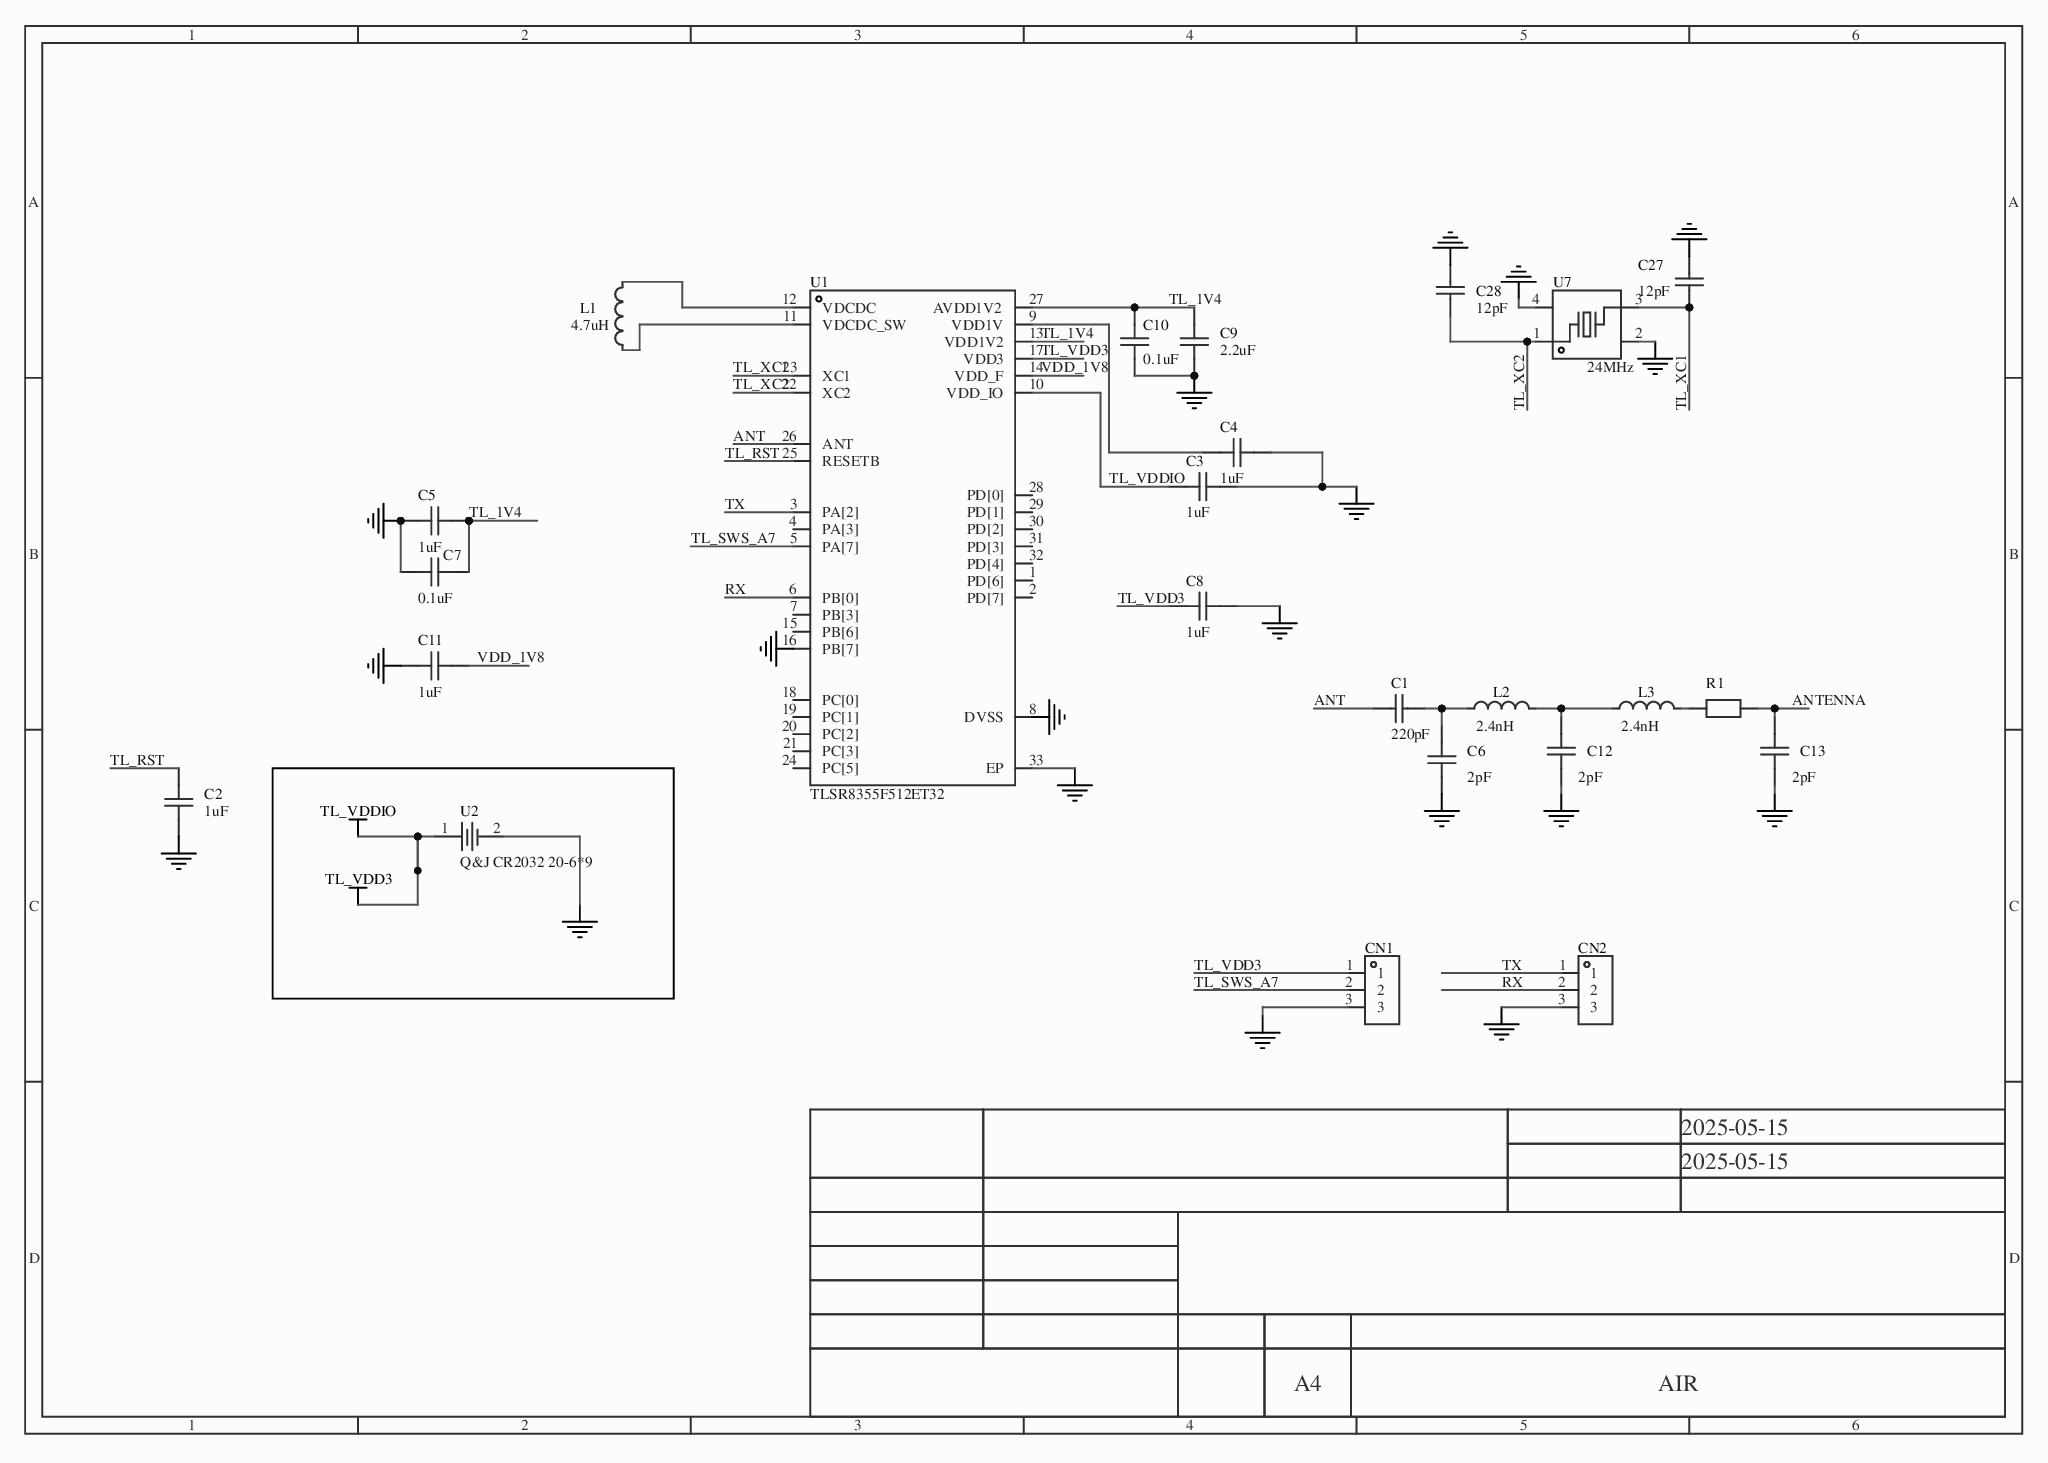
[diagram p0: MISC79017-2.schdoc]
# Altium project MISC79017-6.PrjPCB
1 sheet, 24 parts. Net scope: global (net labels, ports and power ports of the same name join across sheets).
Board file: MISC79017.PcbDoc

## Sheet MISC79017-2.schdoc
size 307 x 218 mm; Version: V1.0; @Page Count: 1; @Update Date: 2025-05-15; @Create Date: 2025-05-15; @Schematic Name: MISC79017; @Page No: 1; @Create Time: 16:34:02; @Update Time: 16:34:04

### Parts
C1  220pF  [C0402]
C2  1uF  [C0402]
C3  1uF  [C0402]
C4  1uF  [C0402]
C5  1uF  [C0402]
C6  2pF  [C0402]
C7  0.1uF  [C0603]
C8  1uF  [C0402]
C9  2.2uF  [C0402]
C10  0.1uF  [C0402]
C11  1uF  [C0402]
C12  2pF  [C0402]
C13  2pF  [C0402]
C27  12pF  [C0402]
C28  12pF  [C0402]
CN1  (no value)  [HDR-TH_3P-P1.27-V-M-A]
CN2  (no value)  [HDR-TH_3P-P1.27-V-M-A]
L1  4.7uH  [IND-SMD_L1.8-W1.2]
L2  2.4nH  [L0402]
L3  2.4nH  [L0402]
R1  (no value)  [R0402]
U1  TLSR8355F512ET32  [TQFN-32_L5.0-W5.0-P0.50-BL-EP3.5]
U2  Q&J CR2032 20-6*9  [BAT-TH_CR2032]
U7  24MHz  [JWT1238]

### Nets
GND: C2.1 C3.1 C4.1 C5.1 C6.1 C7.1 C8.2 C9.1 C10.1 C11.1 C12.1 C13.1 C27.2 C28.2 CN1.3 CN2.3 U1.8(DVSS) U1.16(PB[7]) U1.33(EP) U2.2(-) U7.2(GND) U7.4(GND)
TL_VDD3: C3.2 C8.1 CN1.1 U1.10(VDD_IO) U1.17(VDD3) U2.1(+)  [also labelled TL_VDDIO]
ANT: C1.1 U1.26(ANT)
ANTENNA: C13.2 R1.2
RX: CN2.2 U1.6(PB[0])
TL_1V4: C5.2 C7.2 C9.2 C10.2 U1.13(VDD1V2) U1.27(AVDD1V2)
TL_RST: C2.2 U1.25(RESETB)
TL_SWS_A7: CN1.2 U1.5(PA[7])
TL_XC1: C27.1 U1.23(XC1) U7.3
TL_XC2: C28.1 U1.22(XC2) U7.1
TX: CN2.1 U1.3(PA[2])
VDD_1V8: C11.2 U1.14(VDD_F)
NetC1_2: C1.2 C6.2 L2.1
NetC4_2: C4.2 U1.9(VDD1V)
NetC12_2: C12.2 L2.2 L3.1
NetL1_1: L1.1 U1.11(VDCDC_SW)
NetL1_2: L1.2 U1.12(VDCDC)
NetL3_2: L3.2 R1.1

Not connected (* = marked no-connect by the designer): U1 1(PD[6])* 2(PD[7])* 4(PA[3])* 7(PB[3])* 15(PB[6])* 18(PC[0])* 19(PC[1])* 20(PC[2])* 21(PC[3])* 24(PC[5])* 28(PD[0])* 29(PD[1])* 30(PD[2])* 31(PD[3])* 32(PD[4])*

### Notes on the sheet
- 1
- 2
- 3
- 4
- 5
- 6
- A
- B
- C
- 2025-05-15
- D
- A4
- AIR

### Library data of the parts
C1 = CC0402KRX7R9BB221: Add into BOM: yes; Voltage Rated: 50V; Temperature Coefficient: X7R; Symbol: CC0402KRX7R9BB221; Device: CC0402KRX7R9BB221; Supplier Part: C107025; Manufacturer Part: CC0402KRX7R9BB221; Supplier Footprint: 0402; Datasheet: https://atta.szlcsc.com/upload/public/pdf/source/20170914/C128857_1505359892143968080.pdf; Supplier: LCSC; Convert to PCB: yes; Value: 220pF
C2-C5 C8-C11 = CL05A105KA5NQNC: Add into BOM: yes; Voltage Rated: 25V; Temperature Coefficient: X5R; Symbol: CL05A105KA5NQNC; Device: CL05A105KA5NQNC; Manufacturer Part: CL05A105KA5NQNC; Supplier Footprint: 0402; Datasheet: https://atta.szlcsc.com/upload/public/pdf/source/20160218/1457707763339.pdf; Supplier: LCSC; Convert to PCB: yes
  C2-C5 C8 C11: Supplier Part: C52923; Value: 1uF
  C9: Value: 2.2uF
  C10: Value: 0.1uF
C6 C12 C13 = CC0402CRNPO9BN2R0: Add into BOM: yes; Voltage Rated: 50V; Temperature Coefficient: NP0; Symbol: CC0402CRNPO9BN2R0; Device: CC0402CRNPO9BN2R0; LCSC Part Name: 2pF 50V; Supplier Part: C325454; Manufacturer Part: CC0402CRNPO9BN2R0; Supplier Footprint: 0402; Datasheet: https://atta.szlcsc.com/upload/public/pdf/source/20181031/C325454_B7E70B15058089EBAF4951E75AE2AD52.pdf; Supplier: LCSC; Convert to PCB: yes; Value: 2pF
C7 = CAP_0603: Symbol: CapAcitance; Convert to PCB: yes; Device: CAP_0603; Add into BOM: yes; Supplier Footprint: 0603; Value: 0.1uF
C27 C28 = 0402CG120J500NT: Add into BOM: yes; Voltage Rated: 50V; Temperature Coefficient: C0G; Symbol: 0402CG120J500NT; Device: 0402CG120J500NT; Supplier Part: C1547; Manufacturer Part: 0402CG120J500NT; Supplier Footprint: 0402; Datasheet: https://atta.szlcsc.com/upload/public/pdf/source/20200305/C486355_26A10D38EF8C2A5C37091D0039909270.pdf; Supplier: LCSC; Convert to PCB: yes; Value: 12pF
CN1 CN2 = 3Pin_1.27___: Add into BOM: yes; Supplier Part: C9900016311; Supplier: LCSC; Convert to PCB: yes
L1 = SLC1608F4R7KTT: Add into BOM: yes; Rated Current: 400mA; Symbol: SLC1608F4R7KTT; Device: SLC1608F4R7KTT; Supplier Part: C411909; Manufacturer Part: SLC1608F4R7KTT; Supplier Footprint: SMD,1.8x1.2mm; Datasheet: https://atta.szlcsc.com/upload/public/pdf/source/20190822/C411909_D8F21CE75389351171F329DA46ED7C51.pdf; Supplier: LCSC; Convert to PCB: yes; Value: 4.7uH; Saturation Current (Isat): -; Q @ Freq: -; Frequency - Self Resonant: -; Ratings: -
L2 L3 = LQG15HH2N4S02D: Add into BOM: yes; Rated Current: 300mA; Q @ Freq: 8@100MHz; Frequency - Self Resonant: 6GHz; Symbol: LQG15HH2N4S02D; Device: LQG15HH2N4S02D; LCSC Part Name: 2.4nH; Supplier Part: C602035; Manufacturer Part: LQG15HH2N4S02D; Supplier Footprint: 0402; Datasheet: https://atta.szlcsc.com/upload/public/pdf/source/20190906/C426650_6C25041EF2EDD01B4762A59734016F86.pdf; Supplier: LCSC; Convert to PCB: yes; Value: 2.4nH; Tolerance: -; Saturation Current (Isat): -; Ratings: -
R1 = SCR0402J0R: Add into BOM: yes; Power(Watts): 62.5mW; Overload Voltage (Max): 50V; Symbol: SCR0402J0R; Device: SCR0402J0R; Supplier Part: C3017451; Manufacturer Part: SCR0402J0R; Supplier Footprint: 0402; Datasheet: https://atta.szlcsc.com/upload/public/pdf/source/20220513/247AF9639BA21CF93567DC289CCC6A22.pdf; Supplier: LCSC; Convert to PCB: yes
U1 = TLSR8355F512ET32: Add into BOM: yes; Symbol: TLSR8355F512ET32; Device: TLSR8355F512ET32; LCSC Part Name: TLSR8355F512ET32; Supplier Part: C9900183748; Manufacturer Part: TLSR8355F512ET32; Supplier Footprint: QFN32; Supplier: LCSC; Convert to PCB: yes
U2 = Q&J CR2032 20-6*9: Add into BOM: yes; voltage: 3V; capacity: 240mAh; Device: Q&J CR2032 20-6*9; Supplier Part: C70382; Manufacturer: Q&J; Manufacturer Part: Q&J CR2032 20-6*9; Supplier Footprint: -; Datasheet: https://atta.szlcsc.com/upload/public/pdf/source/20170428/1493376822625.pdf; Supplier: LCSC; Convert to PCB: yes; battery model: -; Type of electrolyte: -
U7 = JWT1238: Add into BOM: yes; Load Capacitance: 12pF; Symbol: JWT1238; Device: JWT1238; Supplier Part: JWT1238; Manufacturer Part: JWT1238; Supplier Footprint: SMD3225-4P; Datasheet: https://atta.szlcsc.com/upload/public/pdf/source/20230620/7CAD71A3C723670283B3D79A2DD7F676.pdf; Supplier: LCSC; Convert to PCB: yes; Value: 24MHz